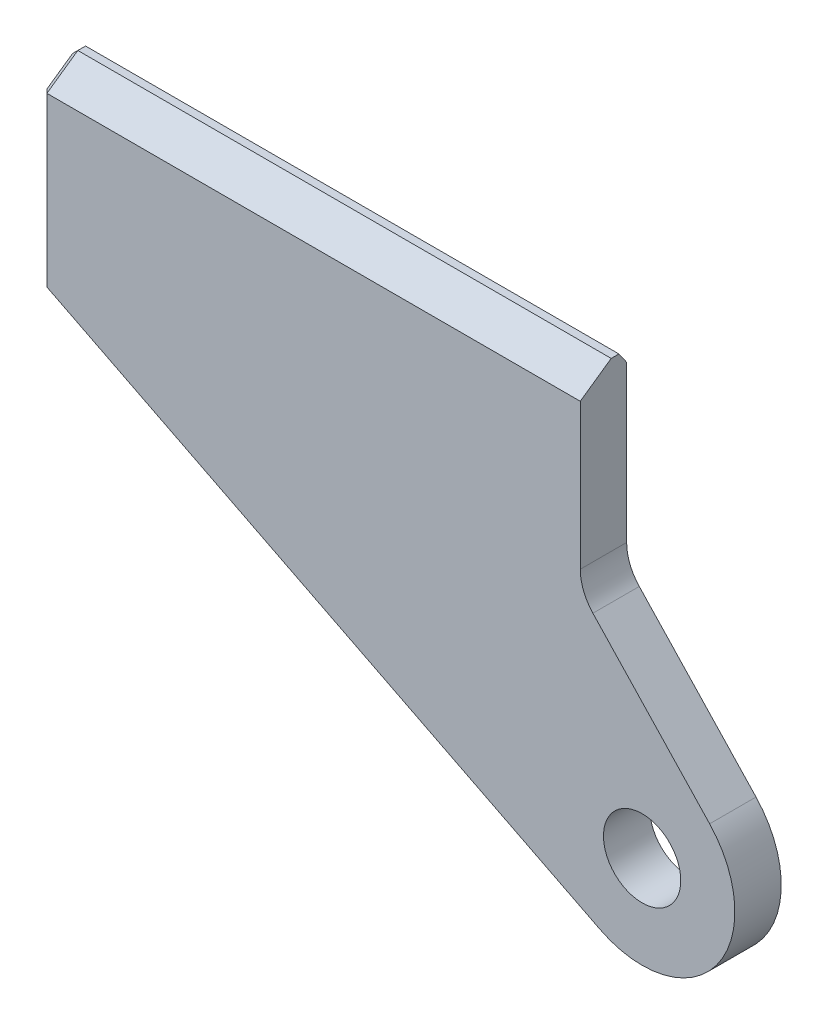
from build123d import *

# Parameters (mm, degrees)
SKETCH_1_R          = 25
EXTRUDE_1_DEPTH     = 30
CUT_EXTRUDE_2_DEPTH = 516.654923374
CUT_EXTRUDE_3_DEPTH = 516.654923374
CHAMFER_1_SIZE      = 5
FILLET_2_R          = 30


with BuildPart() as part:
    # 草图1 → 凸台-拉伸1 (new body)
    with BuildSketch(Plane.XY):
        with BuildLine():
            Line((-40, 250), (-390, 250))
            Line((-390, 250), (-390, 130))
            Line((-390, 130), (-27.078184069, -53.542244514))
            ThreePointArc((-27.078184069, -53.542244514), (48.059978328, -35.919889798), (43.681693947, 41.132828907))
            Line((43.681693947, 41.132828907), (-40, 130))
            Line((-40, 130), (-40, 250))
        make_face()
        Circle(SKETCH_1_R, mode=Mode.SUBTRACT)
    extrude(amount=EXTRUDE_1_DEPTH)

    # 草图2 → 切除-拉伸2 (cut, through all)
    with BuildSketch(Plane(origin=(60, 0, 0), x_dir=(0, 0, -1), z_dir=(1, 0, 0))):
        Polygon((-10, 250), (-30, 235.995849236), (-30, 250), align=None)
    extrude(amount=-CUT_EXTRUDE_2_DEPTH, mode=Mode.SUBTRACT)

    # 草图3 → 切除-拉伸3 (cut, through all)
    with BuildSketch(Plane(origin=(60, 0, 0), x_dir=(0, 0, -1), z_dir=(1, 0, 0))):
        Polygon((-5, 250), (0, 242.859259966), (0, 250), align=None)
    extrude(amount=-CUT_EXTRUDE_3_DEPTH, mode=Mode.SUBTRACT)

    # 倒角1
    chamfer_1_edges = [part.edges().sort_by_distance(p)[0] for p in [
        (-390, 182.997924618, 30),
        (-390, 250, 7.5),
        (-390, 242.997924618, 20),
        (-390, 186.429629983, 0),
        (-390, 246.429629983, 2.5),
    ]]
    chamfer(chamfer_1_edges, length=CHAMFER_1_SIZE)

    # 圆角2
    fillet_2_edges = [part.edges().sort_by_distance(p)[0] for p in [
        (-40, 130, 15),
    ]]
    fillet(fillet_2_edges, radius=FILLET_2_R)


solid = part.part
